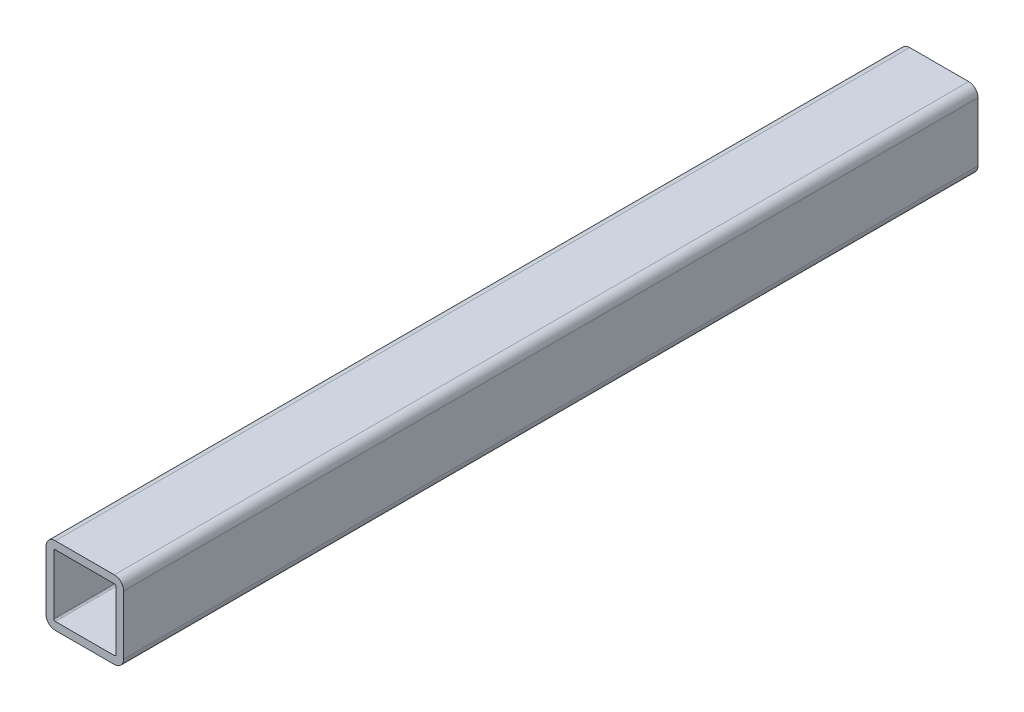
SolidWorks part; units mm, degrees
material "Q235B"
ref_plane "Front Plane" through (0, 0, 0) normal (0, 0, 1) x (1, 0, 0)
ref_plane "Top Plane" through (0, 0, 0) normal (0, 1, 0) x (1, 0, 0)
ref_plane "Right Plane" through (0, 0, 0) normal (1, 0, 0) x (0, 0, -1)
sketch "Sketch1" plane through (0, 0, 0) normal (0, 0, 1) x (1, 0, 0)
  line L0 (6, 45) -> (44, 45)
  line L1 (6, 0) -> (44, 0)
  line L2 (0, 6) -> (0, 44)
  line L3 (6, 50) -> (44, 50)
  line L4 (50, 6) -> (50, 44)
  line L5 (45, 6) -> (45, 44)
  line L6 (6, 5) -> (44, 5)
  line L7 (5, 6) -> (5, 44)
  arc A0 (6, 0) -> (0, 6) centre (6, 6) cw
  arc A1 (44, 0) -> (50, 6) centre (44, 6) ccw
  arc A2 (44, 50) -> (50, 44) centre (44, 44) cw
  arc A3 (0, 44) -> (6, 50) centre (6, 44) cw
  arc A4 (5, 44) -> (6, 45) centre (6, 44) cw
  arc A5 (44, 45) -> (45, 44) centre (44, 44) cw
  arc A6 (44, 5) -> (45, 6) centre (44, 6) ccw
  arc A7 (6, 5) -> (5, 6) centre (6, 6) cw
  point P7 (0, 0)
  point P12 (50, 50)
  point P15 (0, 50)
  dimension "D3" = 6
  dimension "D1" = 50
  dimension "D2" = 50
  dimension "D4" = 5
extrude "Boss-Extrude1" add sketch "Sketch1" along normal blind 550
